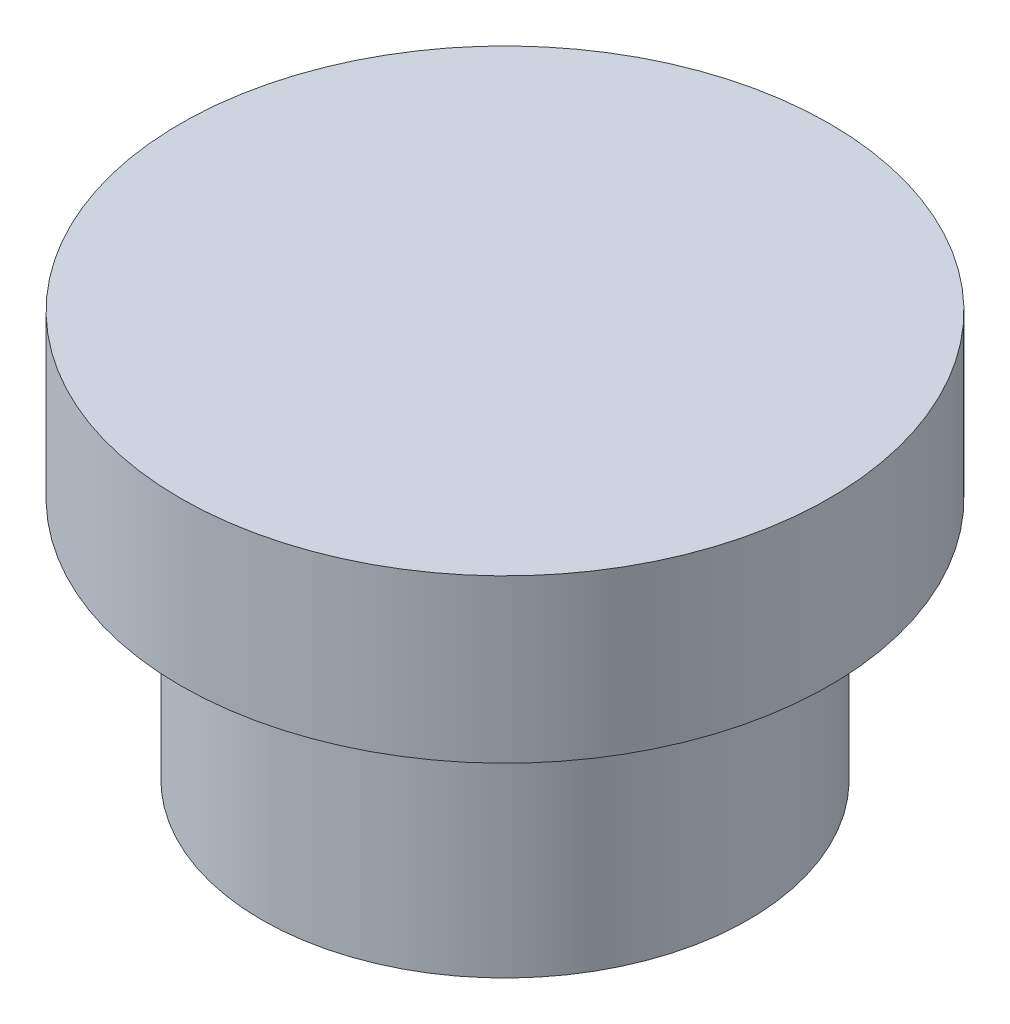
from build123d import *


with BuildPart() as part:
    # Sketch1 → Revolve1 (revolve)
    with BuildSketch(Plane.XY, mode=Mode.PRIVATE) as revolve1_sk:
        Polygon((0, 0), (4, 0), (4, -2), (3, -2), (3, -5), (0, -5), align=None)
    revolve(revolve1_sk.sketch.rotate(Axis((0, -5, 0), (0, 1, 0)), 90), axis=Axis((0, -5, 0), (0, 1, 0)))


solid = part.part
